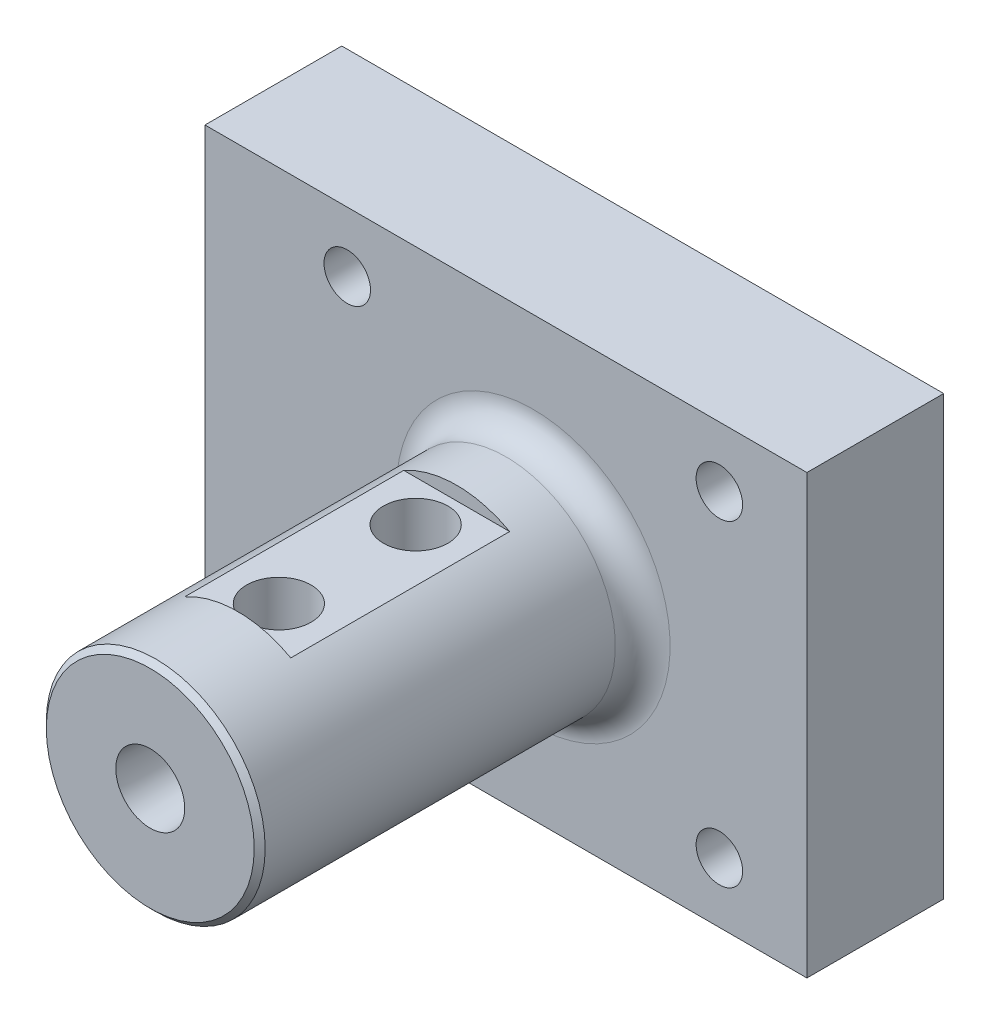
from build123d import *

# Parameters (mm, degrees)
SKETCH_13_W                 = 100
SKETCH_13_H                 = 80
EXTRUDE_3_DEPTH             = 25
SKETCH_14_R                 = 0.5
CUT_EXTRUDE_4_DEPTH         = 18
SKETCH_15_R                 = 20
EXTRUDE_4_DEPTH             = 70
HOLE_WIZARD_10_0_10_1_D     = 10
HOLE_WIZARD_10_0_10_1_DEPTH = 25
HOLE_WIZARD_10_0_10_1_TIP   = 3.004303095
SKETCH_21_OUTSIDE_W         = 133.89
SKETCH_21_OUTSIDE_H         = 113.89
SKETCH_21_OUTSIDE_W_2       = 54.577135948
SKETCH_21_OUTSIDE_H_2       = 35
CUT_EXTRUDE_5_DEPTH         = 40
HOLE_WIZARD_G1_4_1_D        = 11.8
HOLE_WIZARD_G1_4_1_DEPTH    = 25
HOLE_WIZARD_G1_4_1_TIP      = 3.545077652
CHAMFER_1_SIZE              = 1
HOLE_WIZARD_M10_1_D         = 8.5
HOLE_WIZARD_M10_1_DEPTH     = 27.5
HOLE_WIZARD_M10_1_TIP       = 2.553657631
FILLET_1_R                  = 5
HOLE_WIZARD_M6_1_D          = 5
HOLE_WIZARD_M6_1_DEPTH      = 35
HOLE_WIZARD_M6_1_TIP        = 1.502151548
SKETCH_29_W                 = 25
SKETCH_29_H                 = 80
EXTRUDE_5_DEPTH             = 10
HOLE_WIZARD_M10_2_D         = 8.5
HOLE_WIZARD_M10_2_DEPTH     = 27.5
HOLE_WIZARD_M10_2_TIP       = 2.553657631


with BuildPart() as part:
    # 草图13 → 凸台-拉伸3 (new body)
    with BuildSketch(Plane.XY):
        Rectangle(SKETCH_13_W, SKETCH_13_H)
    extrude(amount=EXTRUDE_3_DEPTH)

    # 草图14 → 切除-拉伸4 (cut)
    with BuildSketch(Plane.XY.offset(25)):
        with Locations((-34, 29)):
            Circle(SKETCH_14_R)
        with Locations((34, 29)):
            Circle(SKETCH_14_R)
        with Locations((34, -29)):
            Circle(SKETCH_14_R)
        with Locations((-34, -29)):
            Circle(SKETCH_14_R)
    extrude(amount=-CUT_EXTRUDE_4_DEPTH, mode=Mode.SUBTRACT)

    # 草图15 → 凸台-拉伸4 (add)
    with BuildSketch(Plane.XY.offset(25)):
        with Locations(Location((0, 0, 0), (0, 0, 180))):
            Circle(SKETCH_15_R)
    extrude(amount=EXTRUDE_4_DEPTH)

    # Ø10.0 (10) 直径孔1
    with Locations(Plane.XY.offset(95)):
        with Locations((0, 0)):
            Hole(HOLE_WIZARD_10_0_10_1_D / 2, depth=HOLE_WIZARD_10_0_10_1_DEPTH)
            with Locations((0, 0, -(HOLE_WIZARD_10_0_10_1_DEPTH + HOLE_WIZARD_10_0_10_1_TIP / 2))):  # 118° drill point
                Cone(0, HOLE_WIZARD_10_0_10_1_D / 2, HOLE_WIZARD_10_0_10_1_TIP, mode=Mode.SUBTRACT)

    # 草图19 → 切除-旋转10 (revolve, cut)
    with BuildSketch(Plane(origin=(0, 0, 0), x_dir=(1, 0, 0), z_dir=(0, 1, 0)), mode=Mode.PRIVATE) as cut_revolve_10_sk:
        Polygon((-6.3, -95), (-5.65, -82), (-5, -82), (-5, -95), align=None)
    revolve(cut_revolve_10_sk.sketch.rotate(Axis((0, 0, 95), (0, 0, -1)), 180), axis=Axis((0, 0, 95), (0, 0, -1)), mode=Mode.SUBTRACT)

    # 草图21 outside → 切除-拉伸5 (cut)
    with BuildSketch(Plane.XY.offset(79)):
        Rectangle(SKETCH_21_OUTSIDE_W, SKETCH_21_OUTSIDE_H)
        Rectangle(SKETCH_21_OUTSIDE_W_2, SKETCH_21_OUTSIDE_H_2, mode=Mode.SUBTRACT)
    extrude(amount=-CUT_EXTRUDE_5_DEPTH, mode=Mode.SUBTRACT)

    # G1/4 螺纹孔1
    with Locations(Plane(origin=(0, 17.5, 0), x_dir=(1, 0, 0), z_dir=(0, 1, 0))):
        with Locations((0, -71.5), (0, -46.5)):
            Hole(HOLE_WIZARD_G1_4_1_D / 2, depth=HOLE_WIZARD_G1_4_1_DEPTH)
            with Locations((0, 0, -(HOLE_WIZARD_G1_4_1_DEPTH + HOLE_WIZARD_G1_4_1_TIP / 2))):  # 118° drill point
                Cone(0, HOLE_WIZARD_G1_4_1_D / 2, HOLE_WIZARD_G1_4_1_TIP, mode=Mode.SUBTRACT)

    # 倒角1
    chamfer_1_edges = [part.edges().sort_by_distance(p)[0] for p in [
        (20, 0, 95),
    ]]
    chamfer(chamfer_1_edges, length=CHAMFER_1_SIZE)

    # M10 螺纹孔1
    with Locations(Plane.XY.offset(25)):
        with Locations((-34, 29), (34, 29), (34, -29), (-34, -29)):
            Hole(HOLE_WIZARD_M10_1_D / 2, depth=HOLE_WIZARD_M10_1_DEPTH)
            with Locations((0, 0, -(HOLE_WIZARD_M10_1_DEPTH + HOLE_WIZARD_M10_1_TIP / 2))):  # 118° drill point
                Cone(0, HOLE_WIZARD_M10_1_D / 2, HOLE_WIZARD_M10_1_TIP, mode=Mode.SUBTRACT)

    # 圆角1
    fillet_1_edges = [part.edges().sort_by_distance(p)[0] for p in [
        (20, 0, 25),
    ]]
    fillet(fillet_1_edges, radius=FILLET_1_R)

    # M6 螺纹孔1
    with Locations(Plane.XY.offset(69)):
        with Locations((0, 0)):
            Hole(HOLE_WIZARD_M6_1_D / 2, depth=HOLE_WIZARD_M6_1_DEPTH)
            with Locations((0, 0, -(HOLE_WIZARD_M6_1_DEPTH + HOLE_WIZARD_M6_1_TIP / 2))):  # 118° drill point
                Cone(0, HOLE_WIZARD_M6_1_D / 2, HOLE_WIZARD_M6_1_TIP, mode=Mode.SUBTRACT)

    # 草图29 → 凸台-拉伸5 (add)
    with BuildSketch(Plane.ZY.offset(50)):
        with Locations((12.5, 0)):
            Rectangle(SKETCH_29_W, SKETCH_29_H)
    extrude(amount=EXTRUDE_5_DEPTH)

    # M10 螺纹孔2
    with Locations(Plane.ZY.offset(60)):
        with Locations((12.5, -18), (12.5, 18)):
            Hole(HOLE_WIZARD_M10_2_D / 2, depth=HOLE_WIZARD_M10_2_DEPTH)
            with Locations((0, 0, -(HOLE_WIZARD_M10_2_DEPTH + HOLE_WIZARD_M10_2_TIP / 2))):  # 118° drill point
                Cone(0, HOLE_WIZARD_M10_2_D / 2, HOLE_WIZARD_M10_2_TIP, mode=Mode.SUBTRACT)


solid = part.part
